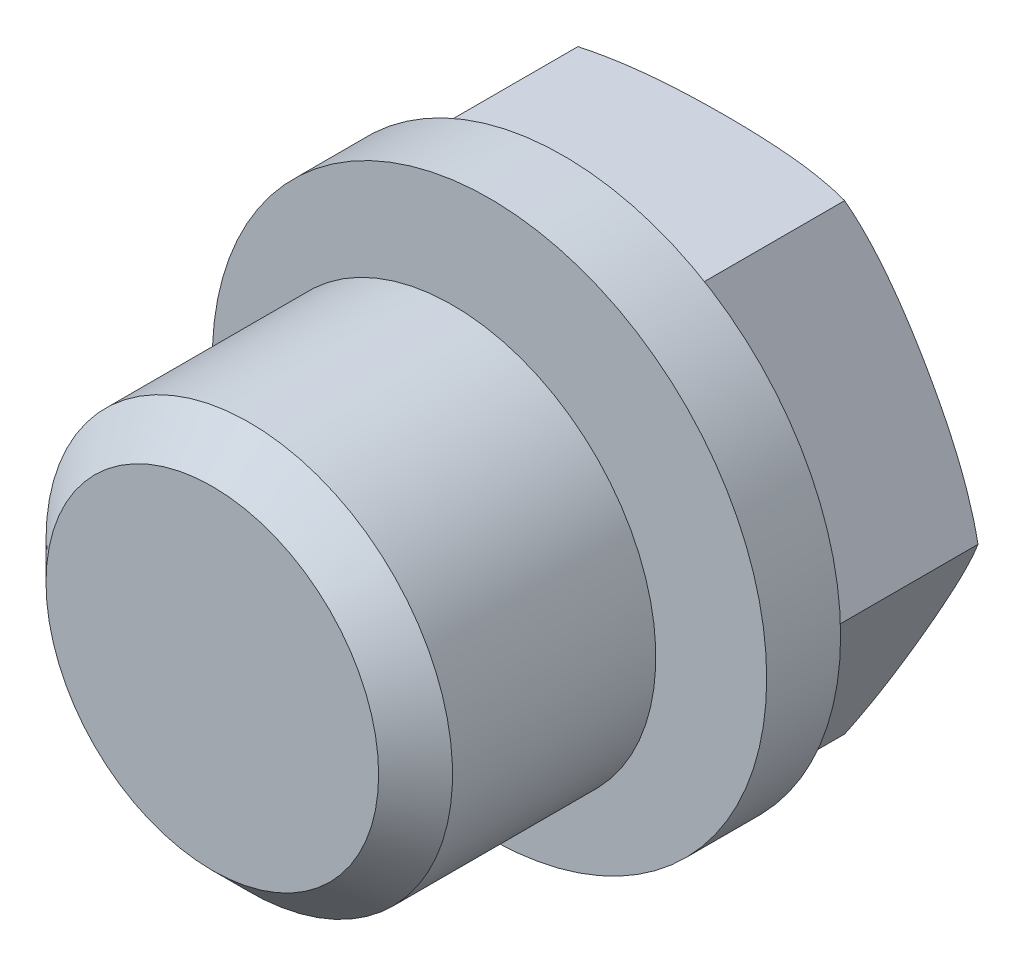
SolidWorks part; units mm, degrees
ref_plane "Front" through (0, 0, 0) normal (0, 0, 1) x (1, 0, 0)
ref_plane "Top" through (0, 0, 0) normal (0, 1, 0) x (1, 0, 0)
ref_plane "Right" through (0, 0, 0) normal (1, 0, 0) x (0, 0, -1)
sketch "Sketch1" plane through (0, 0, 0) normal (0, 0, 1) x (1, 0, 0)
  line L1 (14.4338, 0) -> (7.2169, 12.5)
  line L2 (7.2169, 12.5) -> (-7.2169, 12.5)
  line L3 (-7.2169, 12.5) -> (-14.4338, 0)
  line L4 (-14.4338, 0) -> (-7.2169, -12.5)
  line L5 (-7.2169, -12.5) -> (7.2169, -12.5)
  line L6 (7.2169, -12.5) -> (14.4338, 0)
  circle A0 centre (0, 0) radius 12.5 construction
  dimension "D1" = 25
extrude "Boss-Extrude1" add sketch "Sketch1" along normal blind 9
sketch "Sketch2" plane through (0, 0, 9) normal (0, 0, 1) x (1, 0, 0)
  circle A0 centre (0, 0) radius 15
  dimension "D1" = 30
extrude "Boss-Extrude2" add sketch "Sketch2" along normal blind 4
sketch "Sketch3" plane through (0, 0, 13) normal (0, 0, 1) x (1, 0, 0)
  circle A0 centre (0, 0) radius 7.5
  dimension "D1" = 15
extrude "Boss-Extrude3" add sketch "Sketch3" along normal blind 2
sketch "Sketch4" plane through (0, 0, 15) normal (0, 0, 1) x (1, 0, 0)
  circle A0 centre (0, 0) radius 11
  dimension "D1" = 22
extrude "Boss-Extrude5" add sketch "Sketch4" along normal blind 13
chamfer "Chamfer1" distance 2 angle 45 1 edges at (11, 0, 28)
sketch "Sketch6" plane through (0, 0, 0) normal (0, 1, 0) x (1, 0, 0)
  line L0 (-10.4338, 0) -> (-11.3007, 3.4548)
  line L1 (-14.4338, 0) -> (-14.4338, -1)
  line L2 (-14.4338, -9) -> (-14.4338, 0) construction
  line L3 (0, 0) -> (0, 6.2187) construction
  line L5 (-11.3007, 3.4548) -> (-14.4338, 0)
  arc A0 (-10.4338, 0) -> (-14.4338, -1) centre (-10.559, -7.999) ccw
  dimension "D3" = 8
  dimension "D1" = 1
revolve "Cut-Revolve4" cut sketch "Sketch6" angle 360 about L3
scale "Scale 1" bodies to scale 106 scale about centroid uniform scaling yes scale factor 1.875
